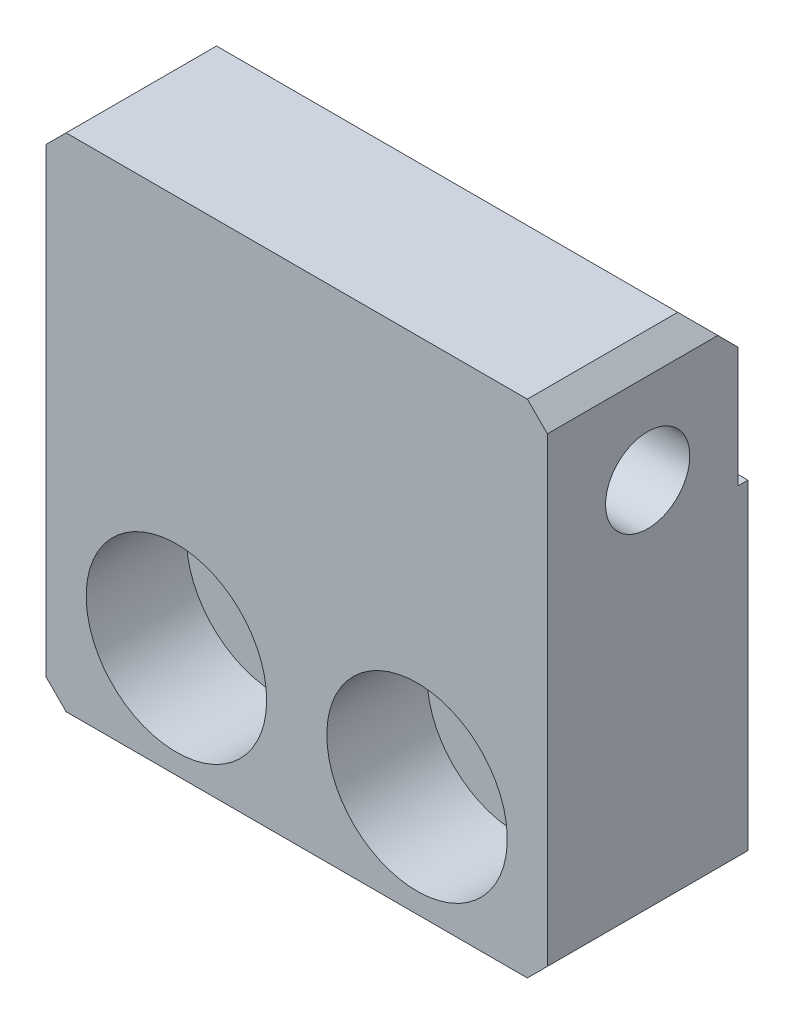
SolidWorks part; units mm, degrees
ref_plane "Front Plane" through (0, 0, 0) normal (0, 0, 1) x (1, 0, 0)
ref_plane "Top Plane" through (0, 0, 0) normal (0, 1, 0) x (1, 0, 0)
ref_plane "Right Plane" through (0, 0, 0) normal (1, 0, 0) x (0, 0, -1)
sketch "Sketch1" plane through (0, 0, 0) normal (0, 0, 1) x (1, 0, 0)
  line L1 (-12.5, 12.5) -> (12.5, 12.5)
  line L2 (-12.5, 12.5) -> (-12.5, -12.5)
  line L3 (-12.5, -12.5) -> (12.5, -12.5)
  line L4 (12.5, 12.5) -> (12.5, -12.5)
  line L5 (-12.5, 12.5) -> (12.5, -12.5) construction
  line L6 (-12.5, -12.5) -> (12.5, 12.5) construction
  point P0 (0, 0)
  dimension "D1" = 25
  dimension "D2" = 25
extrude "Boss-Extrude1" add sketch "Sketch1" along normal blind 10
sketch "Sketch3" plane through (0, 0, 10) normal (0, 0, 1) x (1, 0, 0)
  line L0 (0, 0) -> (0, -50000) construction
  line L1 (-12.5, -12.5) -> (12.5, -12.5) construction
  circle A0 centre (-6, -7) radius 4.5
  circle A1 centre (6, -7) radius 4.5
  dimension "D1" = 12
  dimension "D2" = 9
  dimension "D3" = 5.5
extrude "Cut-Extrude2" cut sketch "Sketch3" against normal blind 5
sketch "Sketch4" plane through (0, 0, 10) normal (0, 0, 1) x (1, 0, 0)
  circle A0 centre (-6, -7) radius 2.25
  circle A1 centre (6, -7) radius 2.25
  dimension "D1" = 4.5
extrude "Cut-Extrude3" cut sketch "Sketch4" against normal blind 14
sketch "Sketch5" plane through (-12.5, 0, 0) normal (-1, 0, 0) x (0, 0, 1)
  line L0 (5, 10) -> (5, -49990) construction
  line L1 (10, 12.5) -> (0, 12.5) construction
  line L2 (0, 7) -> (50000, 7) construction
  circle A0 centre (5, 7) radius 0.9059
  point P4 (5, 12.5)
  dimension "D1" = 5.5
extrude "Cut-Extrude4" cut sketch "Sketch5" against normal blind 31
hole_wizard "M5 Tapped Hole1" positions "3DSketch1" profile "Sketch7" tap size "M5" standard "Gb" end condition through all
sketch3d "3DSketch1"
  line L0 (12.5, 7, 5) -> (-12.5, 7, 5) construction
  point P0 (-12.5, 7, 5)
sketch "Sketch7" plane through (-12.5, 7, 5) normal (0, 1, 0) x (0, 0, 1)
  line L0 (0, 0) -> (0, 25)
  line L1 (0, 25) -> (2.1, 25)
  line L2 (2.1, 25) -> (2.1, 0)
  line L5 (2.1, 0) -> (0, 0)
  line L11 (0, -6.35) -> (0, 107.95) construction
  dimension "通孔螺纹孔钻头直径" = 4.2
  dimension "通孔螺纹孔钻头深度" = 25
cosmetic thread "Cosmetic Thread1" parameters "D2"=5
chamfer "Chamfer1" distance 1 angle 45 4 edges at (12.5, -12.5, 5) (-12.5, -12.5, 5) (12.5, 12.5, 5) (-12.5, 12.5, 5)
sketch "Sketch8" plane through (-12.5, 0, 0) normal (-1, 0, 0) x (0, 0, 1)
  line L1 (0, 12.5) -> (0.5, 12.5)
  line L2 (0, 12.5) -> (0, 4.5)
  line L3 (0, 4.5) -> (0.5, 4.5)
  line L4 (0.5, 12.5) -> (0.5, 4.5)
  dimension "D1" = 0.5
  dimension "D2" = 8
extrude "Cut-Extrude5" cut sketch "Sketch8" against normal blind 31
chamfer "Chamfer2" distance 2 angle 45 1 edges at (0, 12.5, 0.5)
